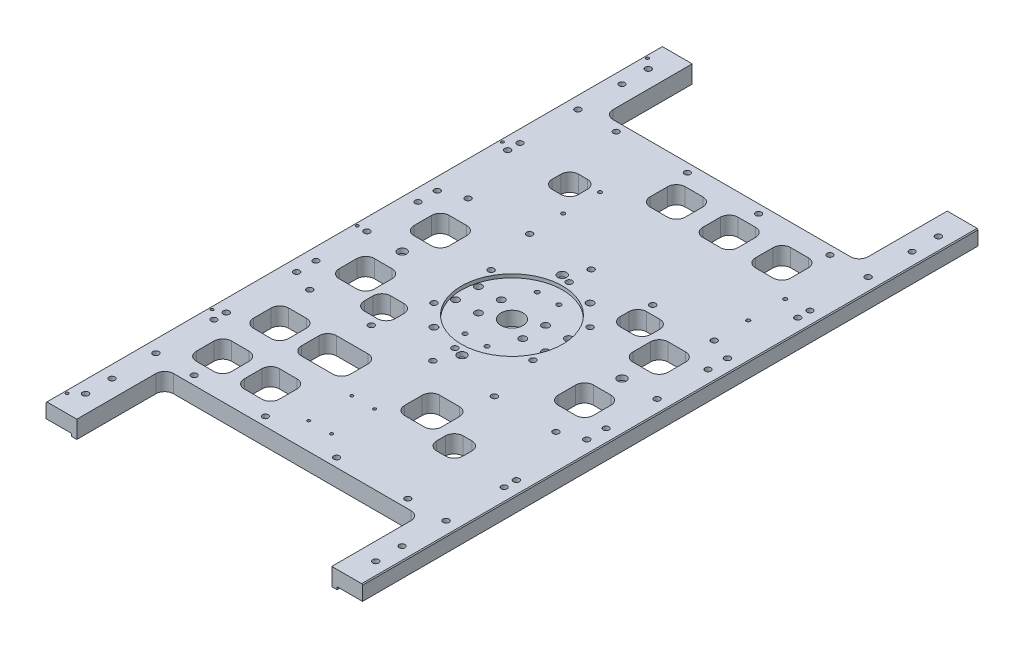
from build123d import *

# Parameters (mm, degrees)
SKETCH_1_W                    = 360
SKETCH_1_H                    = 700
EXTRUDE_1_DEPTH               = 20
SKETCH_2_W                    = 290
SKETCH_2_H                    = 100
CUT_EXTRUDE_1_DEPTH           = 395.081209905
SKETCH_3_W                    = 29
SKETCH_3_H                    = 3
CUT_EXTRUDE_2_DEPTH           = 724.049099301
SKETCH_4_W                    = 29
SKETCH_4_H                    = 3
CUT_EXTRUDE_3_DEPTH           = 724.049099301
SKETCH_5_W                    = 290
SKETCH_5_H                    = 100
CUT_EXTRUDE_4_DEPTH           = 395.081209905
SKETCH_6_W                    = 40
SKETCH_6_H                    = 40
CUT_EXTRUDE_5_DEPTH           = 395.081209905
SKETCH_7_W                    = 40
SKETCH_7_H                    = 40
CUT_EXTRUDE_6_DEPTH           = 395.081209905
SKETCH_8_W                    = 40
SKETCH_8_H                    = 40
CUT_EXTRUDE_7_DEPTH           = 395.081209905
SKETCH_9_W                    = 40
SKETCH_9_H                    = 40
CUT_EXTRUDE_8_DEPTH           = 395.081209905
SKETCH_10_W                   = 40
SKETCH_10_H                   = 40
CUT_EXTRUDE_9_DEPTH           = 395.081209905
SKETCH_11_W                   = 40
SKETCH_11_H                   = 40
CUT_EXTRUDE_10_DEPTH          = 395.081209905
SKETCH_12_W                   = 40
SKETCH_12_H                   = 40
CUT_EXTRUDE_11_DEPTH          = 395.081209905
SKETCH_13_W                   = 40
SKETCH_13_H                   = 40
CUT_EXTRUDE_12_DEPTH          = 395.081209905
SKETCH_14_W                   = 42.291620987
SKETCH_14_H                   = 40
CUT_EXTRUDE_13_DEPTH          = 395.081209905
SKETCH_15_W                   = 55.74271279
SKETCH_15_H                   = 40
CUT_EXTRUDE_14_DEPTH          = 395.081209905
SKETCH_16_W                   = 40
SKETCH_16_H                   = 40
CUT_EXTRUDE_15_DEPTH          = 395.081209905
SKETCH_17_W                   = 40
SKETCH_17_H                   = 40
CUT_EXTRUDE_16_DEPTH          = 395.081209905
SKETCH_18_W                   = 30
SKETCH_18_H                   = 30
CUT_EXTRUDE_17_DEPTH          = 395.081209905
SKETCH_19_W                   = 30
SKETCH_19_H                   = 30
CUT_EXTRUDE_18_DEPTH          = 395.081209905
SKETCH_20_W                   = 35
SKETCH_20_H                   = 30
CUT_EXTRUDE_19_DEPTH          = 395.081209905
SKETCH_21_W                   = 35
SKETCH_21_H                   = 30
CUT_EXTRUDE_20_DEPTH          = 395.081209905
SKETCH_22_W                   = 34
SKETCH_22_H                   = 82
CUT_EXTRUDE_21_DEPTH          = 5
SKETCH_23_W                   = 34
SKETCH_23_H                   = 82
CUT_EXTRUDE_22_DEPTH          = 5
SKETCH_24_W                   = 95
SKETCH_24_H                   = 60
CUT_EXTRUDE_23_DEPTH          = 12
SKETCH_25_W                   = 220
SKETCH_25_H                   = 80
CUT_EXTRUDE_24_DEPTH          = 12
HOLE_WIZARD_4_2_4_2_1_D       = 4.2
HOLE_WIZARD_3_3_3_3_1_D       = 3.3
HOLE_WIZARD_8_0_8_1_D         = 8
HOLE_WIZARD_6_8_6_8_1_D       = 6.8
HOLE_WIZARD_6_8_6_8_1_DEPTH   = 20
HOLE_WIZARD_3_3_3_3_2_D       = 3.3
HOLE_WIZARD_3_3_3_3_2_DEPTH   = 10.1
HOLE_WIZARD_3_3_3_3_2_TIP     = 0.991420021
HOLE_WIZARD_6_8_6_8_2_D       = 6.8
HOLE_WIZARD_M6_1_D            = 6.6
HOLE_WIZARD_M6_1_CBORE_D      = 11
HOLE_WIZARD_M6_1_CBORE_DEPTH  = 6.4
HOLE_WIZARD_M6_2_D            = 6.6
HOLE_WIZARD_M6_2_CBORE_D      = 11
HOLE_WIZARD_M6_2_CBORE_DEPTH  = 6.4
HOLE_WIZARD_M24_1_D           = 25
HOLE_WIZARD_M24_1_CBORE_D     = 115
HOLE_WIZARD_M24_1_CBORE_DEPTH = 4
HOLE_WIZARD_5_0_5_1_D         = 5
HOLE_WIZARD_5_0_5_1_DEPTH     = 20
HOLE_WIZARD_M4_1_D            = 4.5
HOLE_WIZARD_M4_1_DEPTH        = 16
HOLE_WIZARD_M4_1_CBORE_D      = 8
HOLE_WIZARD_M4_1_CBORE_DEPTH  = 6
HOLE_WIZARD_5_0_5_2_D         = 5
HOLE_WIZARD_5_0_5_2_DEPTH     = 15
HOLE_WIZARD_5_0_5_2_TIP       = 1.502151548
CHAMFER_1_SIZE                = 1
FILLET_1_R                    = 5
FILLET_2_R                    = 10


with BuildPart() as part:
    # 草图1 → 凸台-拉伸1 (new body)
    with BuildSketch(Plane.XZ):
        Rectangle(SKETCH_1_W, SKETCH_1_H)
    extrude(amount=-EXTRUDE_1_DEPTH)

    # 草图2 → 切除-拉伸1 (cut, through all)
    with BuildSketch(Plane(origin=(0, 20, 0), x_dir=(-1, 0, 0), z_dir=(0, 1, 0))):
        with Locations((0, 300)):
            Rectangle(SKETCH_2_W, SKETCH_2_H)
    extrude(amount=-CUT_EXTRUDE_1_DEPTH, mode=Mode.SUBTRACT)

    # 草图3 → 切除-拉伸2 (cut, through all)
    with BuildSketch(Plane.XY.offset(350)):
        with Locations((-165.5, 1.5)):
            Rectangle(SKETCH_3_W, SKETCH_3_H)
    extrude(amount=-CUT_EXTRUDE_2_DEPTH, mode=Mode.SUBTRACT)

    # 草图4 → 切除-拉伸3 (cut, through all)
    with BuildSketch(Plane.XY.offset(350)):
        with Locations((165.5, 1.5)):
            Rectangle(SKETCH_4_W, SKETCH_4_H)
    extrude(amount=-CUT_EXTRUDE_3_DEPTH, mode=Mode.SUBTRACT)

    # 草图5 → 切除-拉伸4 (cut, through all)
    with BuildSketch(Plane(origin=(0, 20, 0), x_dir=(-1, 0, 0), z_dir=(0, 1, 0))):
        with Locations((0, -300)):
            Rectangle(SKETCH_5_W, SKETCH_5_H)
    extrude(amount=-CUT_EXTRUDE_4_DEPTH, mode=Mode.SUBTRACT)

    # 草图6 → 切除-拉伸5 (cut, through all)
    with BuildSketch(Plane.XZ):
        with Locations((101.993043785, -205)):
            Rectangle(SKETCH_6_W, SKETCH_6_H)
    extrude(amount=-CUT_EXTRUDE_5_DEPTH, mode=Mode.SUBTRACT)

    # 草图7 → 切除-拉伸6 (cut, through all)
    with BuildSketch(Plane.XZ):
        with Locations((41.993043785, -205)):
            Rectangle(SKETCH_7_W, SKETCH_7_H)
    extrude(amount=-CUT_EXTRUDE_6_DEPTH, mode=Mode.SUBTRACT)

    # 草图8 → 切除-拉伸7 (cut, through all)
    with BuildSketch(Plane.XZ):
        with Locations((125, -42.5)):
            Rectangle(SKETCH_8_W, SKETCH_8_H)
    extrude(amount=-CUT_EXTRUDE_7_DEPTH, mode=Mode.SUBTRACT)

    # 草图9 → 切除-拉伸8 (cut, through all)
    with BuildSketch(Plane.XZ):
        with Locations((-18.006956215, -205)):
            Rectangle(SKETCH_9_W, SKETCH_9_H)
    extrude(amount=-CUT_EXTRUDE_8_DEPTH, mode=Mode.SUBTRACT)

    # 草图10 → 切除-拉伸9 (cut, through all)
    with BuildSketch(Plane.XZ):
        with Locations((125, 42.5)):
            Rectangle(SKETCH_10_W, SKETCH_10_H)
    extrude(amount=-CUT_EXTRUDE_9_DEPTH, mode=Mode.SUBTRACT)

    # 草图11 → 切除-拉伸10 (cut, through all)
    with BuildSketch(Plane.XZ):
        with Locations((-124, 42.5)):
            Rectangle(SKETCH_11_W, SKETCH_11_H)
    extrude(amount=-CUT_EXTRUDE_10_DEPTH, mode=Mode.SUBTRACT)

    # 草图12 → 切除-拉伸11 (cut, through all)
    with BuildSketch(Plane.XZ):
        with Locations((-124, -42.5)):
            Rectangle(SKETCH_12_W, SKETCH_12_H)
    extrude(amount=-CUT_EXTRUDE_11_DEPTH, mode=Mode.SUBTRACT)

    # 草图13 → 切除-拉伸12 (cut, through all)
    with BuildSketch(Plane.XZ):
        with Locations((-69.5, 205)):
            Rectangle(SKETCH_13_W, SKETCH_13_H)
    extrude(amount=-CUT_EXTRUDE_12_DEPTH, mode=Mode.SUBTRACT)

    # 草图14 → 切除-拉伸13 (cut, through all)
    with BuildSketch(Plane.XZ):
        with Locations((48.946531367, 140)):
            Rectangle(SKETCH_14_W, SKETCH_14_H)
    extrude(amount=-CUT_EXTRUDE_13_DEPTH, mode=Mode.SUBTRACT)

    # 草图15 → 切除-拉伸14 (cut, through all)
    with BuildSketch(Plane.XZ):
        with Locations((-61.628643605, 140)):
            Rectangle(SKETCH_15_W, SKETCH_15_H)
    extrude(amount=-CUT_EXTRUDE_14_DEPTH, mode=Mode.SUBTRACT)

    # 草图16 → 切除-拉伸15 (cut, through all)
    with BuildSketch(Plane.XZ):
        with Locations((-124, 205)):
            Rectangle(SKETCH_16_W, SKETCH_16_H)
    extrude(amount=-CUT_EXTRUDE_15_DEPTH, mode=Mode.SUBTRACT)

    # 草图17 → 切除-拉伸16 (cut, through all)
    with BuildSketch(Plane.XZ):
        with Locations((-124, 140)):
            Rectangle(SKETCH_17_W, SKETCH_17_H)
    extrude(amount=-CUT_EXTRUDE_16_DEPTH, mode=Mode.SUBTRACT)

    # 草图18 → 切除-拉伸17 (cut, through all)
    with BuildSketch(Plane.XZ):
        with Locations((-96, -161.667964793)):
            Rectangle(SKETCH_18_W, SKETCH_18_H)
    extrude(amount=-CUT_EXTRUDE_17_DEPTH, mode=Mode.SUBTRACT)

    # 草图19 → 切除-拉伸18 (cut, through all)
    with BuildSketch(Plane.XZ):
        with Locations((96, 161.667964793)):
            Rectangle(SKETCH_19_W, SKETCH_19_H)
    extrude(amount=-CUT_EXTRUDE_18_DEPTH, mode=Mode.SUBTRACT)

    # 草图20 → 切除-拉伸19 (cut, through all)
    with BuildSketch(Plane.XZ):
        with Locations((80.5, -65)):
            Rectangle(SKETCH_20_W, SKETCH_20_H)
    extrude(amount=-CUT_EXTRUDE_19_DEPTH, mode=Mode.SUBTRACT)

    # 草图21 → 切除-拉伸20 (cut, through all)
    with BuildSketch(Plane(origin=(0, 20, 0), x_dir=(-1, 0, 0), z_dir=(0, 1, 0))):
        with Locations((80.5, 65)):
            Rectangle(SKETCH_21_W, SKETCH_21_H)
    extrude(amount=-CUT_EXTRUDE_20_DEPTH, mode=Mode.SUBTRACT)

    # 草图22 → 切除-拉伸21 (cut)
    with BuildSketch(Plane.XZ):
        with Locations((-38.2, 0)):
            Rectangle(SKETCH_22_W, SKETCH_22_H)
    extrude(amount=-CUT_EXTRUDE_21_DEPTH, mode=Mode.SUBTRACT)

    # 草图23 → 切除-拉伸22 (cut)
    with BuildSketch(Plane.XZ):
        with Locations((38.2, 0)):
            Rectangle(SKETCH_23_W, SKETCH_23_H)
    extrude(amount=-CUT_EXTRUDE_22_DEPTH, mode=Mode.SUBTRACT)

    # 草图24 → 切除-拉伸23 (cut)
    with BuildSketch(Plane.XZ):
        with Locations((7.5, 195)):
            Rectangle(SKETCH_24_W, SKETCH_24_H)
    extrude(amount=-CUT_EXTRUDE_23_DEPTH, mode=Mode.SUBTRACT)

    # 草图25 → 切除-拉伸24 (cut)
    with BuildSketch(Plane.XZ):
        with Locations((35, -140)):
            Rectangle(SKETCH_25_W, SKETCH_25_H)
    extrude(amount=-CUT_EXTRUDE_24_DEPTH, mode=Mode.SUBTRACT)

    # 草图26 → 切除-旋转1 (revolve, cut)
    with BuildSketch(Plane(origin=(0, 0, -0.131178393), x_dir=(-1, 0, 0), z_dir=(0, 0, -1)), mode=Mode.PRIVATE) as cut_revolve_1_sk:
        Polygon((-130, 0), (-125, 0), (-125, 20), (-130, 20), (-130, 14.6), (-127.75, 14.6), (-127.75, 6), (-130, 6), align=None)
    revolve(cut_revolve_1_sk.sketch.rotate(Axis((125, 0, -0.131178393), (0, 1, 0)), 270), axis=Axis((125, 0, -0.131178393), (0, 1, 0)), mode=Mode.SUBTRACT)

    # 草图27 → 切除-旋转2 (revolve, cut)
    with BuildSketch(Plane(origin=(0, 0, -0.131178393), x_dir=(-1, 0, 0), z_dir=(0, 0, -1)), mode=Mode.PRIVATE) as cut_revolve_2_sk:
        Polygon((120, 0), (125, 0), (125, 20), (120, 20), (120, 14.6), (122.25, 14.6), (122.25, 6), (120, 6), align=None)
    revolve(cut_revolve_2_sk.sketch.rotate(Axis((-125, 0, -0.131178393), (0, 1, 0)), 270), axis=Axis((-125, 0, -0.131178393), (0, 1, 0)), mode=Mode.SUBTRACT)

    # 草图28 → 切除-旋转3 (revolve, cut)
    with BuildSketch(Plane(origin=(0, 0, -68.131178393), x_dir=(-1, 0, 0), z_dir=(0, 0, -1)), mode=Mode.PRIVATE) as cut_revolve_3_sk:
        Polygon((6, 0), (11, 0), (11, 20), (6, 20), (6, 14.6), (8.25, 14.6), (8.25, 6), (6, 6), align=None)
    revolve(cut_revolve_3_sk.sketch.rotate(Axis((-11, 0, -68.131178393), (0, 1, 0)), 270), axis=Axis((-11, 0, -68.131178393), (0, 1, 0)), mode=Mode.SUBTRACT)

    # 草图29 → 切除-旋转4 (revolve, cut)
    with BuildSketch(Plane(origin=(0, 0, 67.868821607), x_dir=(-1, 0, 0), z_dir=(0, 0, -1)), mode=Mode.PRIVATE) as cut_revolve_4_sk:
        Polygon((-16, 0), (-11, 0), (-11, 20), (-16, 20), (-16, 14.6), (-13.75, 14.6), (-13.75, 6), (-16, 6), align=None)
    revolve(cut_revolve_4_sk.sketch.rotate(Axis((11, 0, 67.868821607), (0, 1, 0)), 270), axis=Axis((11, 0, 67.868821607), (0, 1, 0)), mode=Mode.SUBTRACT)

    # Ø4.2 (4.2) 直径孔1 (through all)
    with Locations(Plane(origin=(0, 12, 0), x_dir=(-1, 0, 0), z_dir=(0, -1, 0))):
        with Locations((71, 171.2), (71, 129.2), (-139.5, 129.2), (-139.5, 171.2)):
            Hole(HOLE_WIZARD_4_2_4_2_1_D / 2)

    # Ø3.3 (3.3) 直径孔1 (through all)
    with Locations(Plane(origin=(0, 12, 0), x_dir=(-1, 0, 0), z_dir=(0, -1, 0))):
        with Locations((11.7, -219.5), (-14.3, -219.5), (11.7, -170.5), (-14.3, -170.5)):
            Hole(HOLE_WIZARD_3_3_3_3_1_D / 2)

    # Ø8.0 (8) 直径孔1 (through all)
    with Locations(Plane(origin=(0, 0, 0), x_dir=(-1, 0, 0), z_dir=(0, -1, 0))):
        with Locations((-32.5, 56.291651246), (32.5, -56.291651246)):
            Hole(HOLE_WIZARD_8_0_8_1_D / 2)

    # Ø6.8 (6.8) 直径孔1
    with Locations(Plane(origin=(0, 20, 0), x_dir=(1, 0, 0), z_dir=(0, 1, 0))):
        with Locations((-165, -320), (-165, -240), (-165, -160), (-165, -80), (-165, 0), (-165, 80), (-165, 160), (-165, 240), (-165, 320), (165, -320), (165, -240), (165, -160), (165, -80), (165, 0), (165, 80), (165, 160), (165, 240), (165, 320)):
            Hole(HOLE_WIZARD_6_8_6_8_1_D / 2, depth=HOLE_WIZARD_6_8_6_8_1_DEPTH)

    # Ø3.3 (3.3) 直径孔2
    with Locations(Plane(origin=(0, 20, 0), x_dir=(1, 0, 0), z_dir=(0, 1, 0))):
        with Locations((-176, 330), (-176, 165), (-176, 0), (-176, -165), (-176, -330)):
            Hole(HOLE_WIZARD_3_3_3_3_2_D / 2, depth=HOLE_WIZARD_3_3_3_3_2_DEPTH)
            with Locations((0, 0, -(HOLE_WIZARD_3_3_3_3_2_DEPTH + HOLE_WIZARD_3_3_3_3_2_TIP / 2))):  # 118° drill point
                Cone(0, HOLE_WIZARD_3_3_3_3_2_D / 2, HOLE_WIZARD_3_3_3_3_2_TIP, mode=Mode.SUBTRACT)

    # Ø6.8 (6.8) 直径孔2 (through all)
    with Locations(Plane(origin=(0, 20, 0), x_dir=(1, 0, 0), z_dir=(0, 1, 0))):
        with Locations((140, -90), (70, -90), (0, -90), (-70, -90), (-140, -90), (56.291651246, -32.5), (0, -65), (-56.291651246, -32.5), (-56.291651246, 32.5), (0, 65), (56.291651246, 32.5), (140, 90), (70, 90), (0, 90), (-70, 90), (-140, 90)):
            Hole(HOLE_WIZARD_6_8_6_8_2_D / 2)

    # M6 六角头螺栓的柱形沉头孔1 (through all)
    with Locations(Plane(origin=(0, 0, 0), x_dir=(-1, 0, 0), z_dir=(0, -1, 0))):
        with Locations((40.5, -240), (-40.5, -240), (-121.5, -240), (121.5, -240), (-121.5, 240), (-40.5, 240), (40.5, 240), (121.5, 240)):
            CounterBoreHole(HOLE_WIZARD_M6_1_D / 2, HOLE_WIZARD_M6_1_CBORE_D / 2, HOLE_WIZARD_M6_1_CBORE_DEPTH)

    # M6 六角头螺栓的柱形沉头孔2 (through all)
    with Locations(Plane(origin=(0, 3, 0), x_dir=(-1, 0, 0), z_dir=(0, -1, 0))):
        with Locations((165, 58), (165, 174), (165, 290), (165, -58), (165, -174), (165, -290), (-165, -290), (-165, -174), (-165, -58), (-165, 58), (-165, 174), (-165, 290)):
            CounterBoreHole(HOLE_WIZARD_M6_2_D / 2, HOLE_WIZARD_M6_2_CBORE_D / 2, HOLE_WIZARD_M6_2_CBORE_DEPTH)

    # M24 六角头螺栓的柱形沉头孔1 (through all)
    with Locations(Plane(origin=(0, 20, 0), x_dir=(1, 0, 0), z_dir=(0, 1, 0))):
        with Locations((0, 0)):
            CounterBoreHole(HOLE_WIZARD_M24_1_D / 2, HOLE_WIZARD_M24_1_CBORE_D / 2, HOLE_WIZARD_M24_1_CBORE_DEPTH)

    # Ø5.0 (5) 直径孔1
    with Locations(Plane(origin=(0, 0, 0), x_dir=(-1, 0, 0), z_dir=(0, -1, 0))):
        with Locations((-12.339130192, 41), (12.339130192, 41), (-12.5, -41), (12.5, -41)):
            Hole(HOLE_WIZARD_5_0_5_1_D / 2, depth=HOLE_WIZARD_5_0_5_1_DEPTH)

    # M4 六角头机械螺钉的柱形沉头孔1
    with Locations(Plane(origin=(0, 16, 0), x_dir=(1, 0, 0), z_dir=(0, 1, 0))):
        with Locations((-51.2, -13), (-25.2, -13), (-25.2, 13), (-51.2, 13), (51.2, -13), (25.2, -13), (25.2, 13), (51.2, 13)):
            CounterBoreHole(HOLE_WIZARD_M4_1_D / 2, HOLE_WIZARD_M4_1_CBORE_D / 2, HOLE_WIZARD_M4_1_CBORE_DEPTH, depth=HOLE_WIZARD_M4_1_DEPTH)

    # Ø5.0 (5) 直径孔2
    with Locations(Plane(origin=(0, 0, 0), x_dir=(-1, 0, 0), z_dir=(0, -1, 0))):
        with Locations((-110.184699076, -215.5), (-110.184699076, -189.5), (-66.184699076, -215.5), (-66.184699076, -189.5), (110.184699076, 215.5), (110.184699076, 189.5), (66.184699076, 215.5), (66.184699076, 189.5)):
            Hole(HOLE_WIZARD_5_0_5_2_D / 2, depth=HOLE_WIZARD_5_0_5_2_DEPTH)
            with Locations((0, 0, -(HOLE_WIZARD_5_0_5_2_DEPTH + HOLE_WIZARD_5_0_5_2_TIP / 2))):  # 118° drill point
                Cone(0, HOLE_WIZARD_5_0_5_2_D / 2, HOLE_WIZARD_5_0_5_2_TIP, mode=Mode.SUBTRACT)

    # 倒角1
    chamfer_1_edges = [part.edges().sort_by_distance(p)[0] for p in [
        (-180, 20, 0),
        (180, 20, 0),
    ]]
    chamfer(chamfer_1_edges, length=CHAMFER_1_SIZE)

    # 圆角1
    fillet_1_edges = [part.edges().sort_by_distance(p)[0] for p in [
        (-21.2, 2.5, -41),
        (-55.2, 2.5, -41),
        (-55.2, 2.5, 41),
        (-21.2, 2.5, 41),
        (21.2, 2.5, 41),
        (55.2, 2.5, 41),
        (55.2, 2.5, -41),
        (21.2, 2.5, -41),
    ]]
    fillet(fillet_1_edges, radius=FILLET_1_R)

    # 圆角2
    fillet_2_edges = [part.edges().sort_by_distance(p)[0] for p in [
        (61.993043785, 10, -185),
        (61.993043785, 10, -225),
        (21.993043785, 10, -225),
        (21.993043785, 10, -185),
        (105, 10, -22.5),
        (145, 10, -22.5),
        (145, 10, -62.5),
        (105, 10, -62.5),
        (1.993043785, 10, -185),
        (1.993043785, 10, -225),
        (-38.006956215, 10, -225),
        (-38.006956215, 10, -185),
        (105, 10, 62.5),
        (145, 10, 62.5),
        (145, 10, 22.5),
        (105, 10, 22.5),
        (-104, 10, 62.5),
        (-104, 10, 22.5),
        (-144, 10, 22.5),
        (-144, 10, 62.5),
        (-144, 10, -62.5),
        (-144, 10, -22.5),
        (-104, 10, -22.5),
        (-104, 10, -62.5),
        (-89.5, 10, 225),
        (-49.5, 10, 225),
        (-49.5, 10, 185),
        (-145, 10, 250),
        (-89.5, 10, 185),
        (145, 10, 250),
        (27.800720873, 10, 160),
        (70.09234186, 10, 160),
        (70.09234186, 10, 120),
        (27.800720873, 10, 120),
        (-33.75728721, 10, 160),
        (-33.75728721, 10, 120),
        (-89.5, 10, 120),
        (-89.5, 10, 160),
        (-104, 10, 225),
        (-104, 10, 185),
        (-144, 10, 185),
        (-144, 10, 225),
        (-104, 10, 160),
        (-104, 10, 120),
        (-144, 10, 120),
        (-144, 10, 160),
        (-81, 10, -146.667964793),
        (-81, 10, -176.667964793),
        (-111, 10, -176.667964793),
        (-111, 10, -146.667964793),
        (81, 10, 146.667964793),
        (81, 10, 176.667964793),
        (111, 10, 176.667964793),
        (111, 10, 146.667964793),
        (63, 10, -80),
        (63, 10, -50),
        (98, 10, -50),
        (98, 10, -80),
        (-63, 10, 80),
        (-98, 10, 80),
        (-98, 10, 50),
        (-63, 10, 50),
        (55, 6, 225),
        (55, 6, 165),
        (-40, 6, 165),
        (-40, 6, 225),
        (145, 6, -100),
        (145, 6, -180),
        (-75, 6, -180),
        (-75, 6, -100),
        (145, 10, -250),
        (-145, 10, -250),
        (81.993043785, 10, -185),
        (121.993043785, 10, -185),
        (121.993043785, 10, -225),
        (81.993043785, 10, -225),
    ]]
    fillet(fillet_2_edges, radius=FILLET_2_R)


solid = part.part
